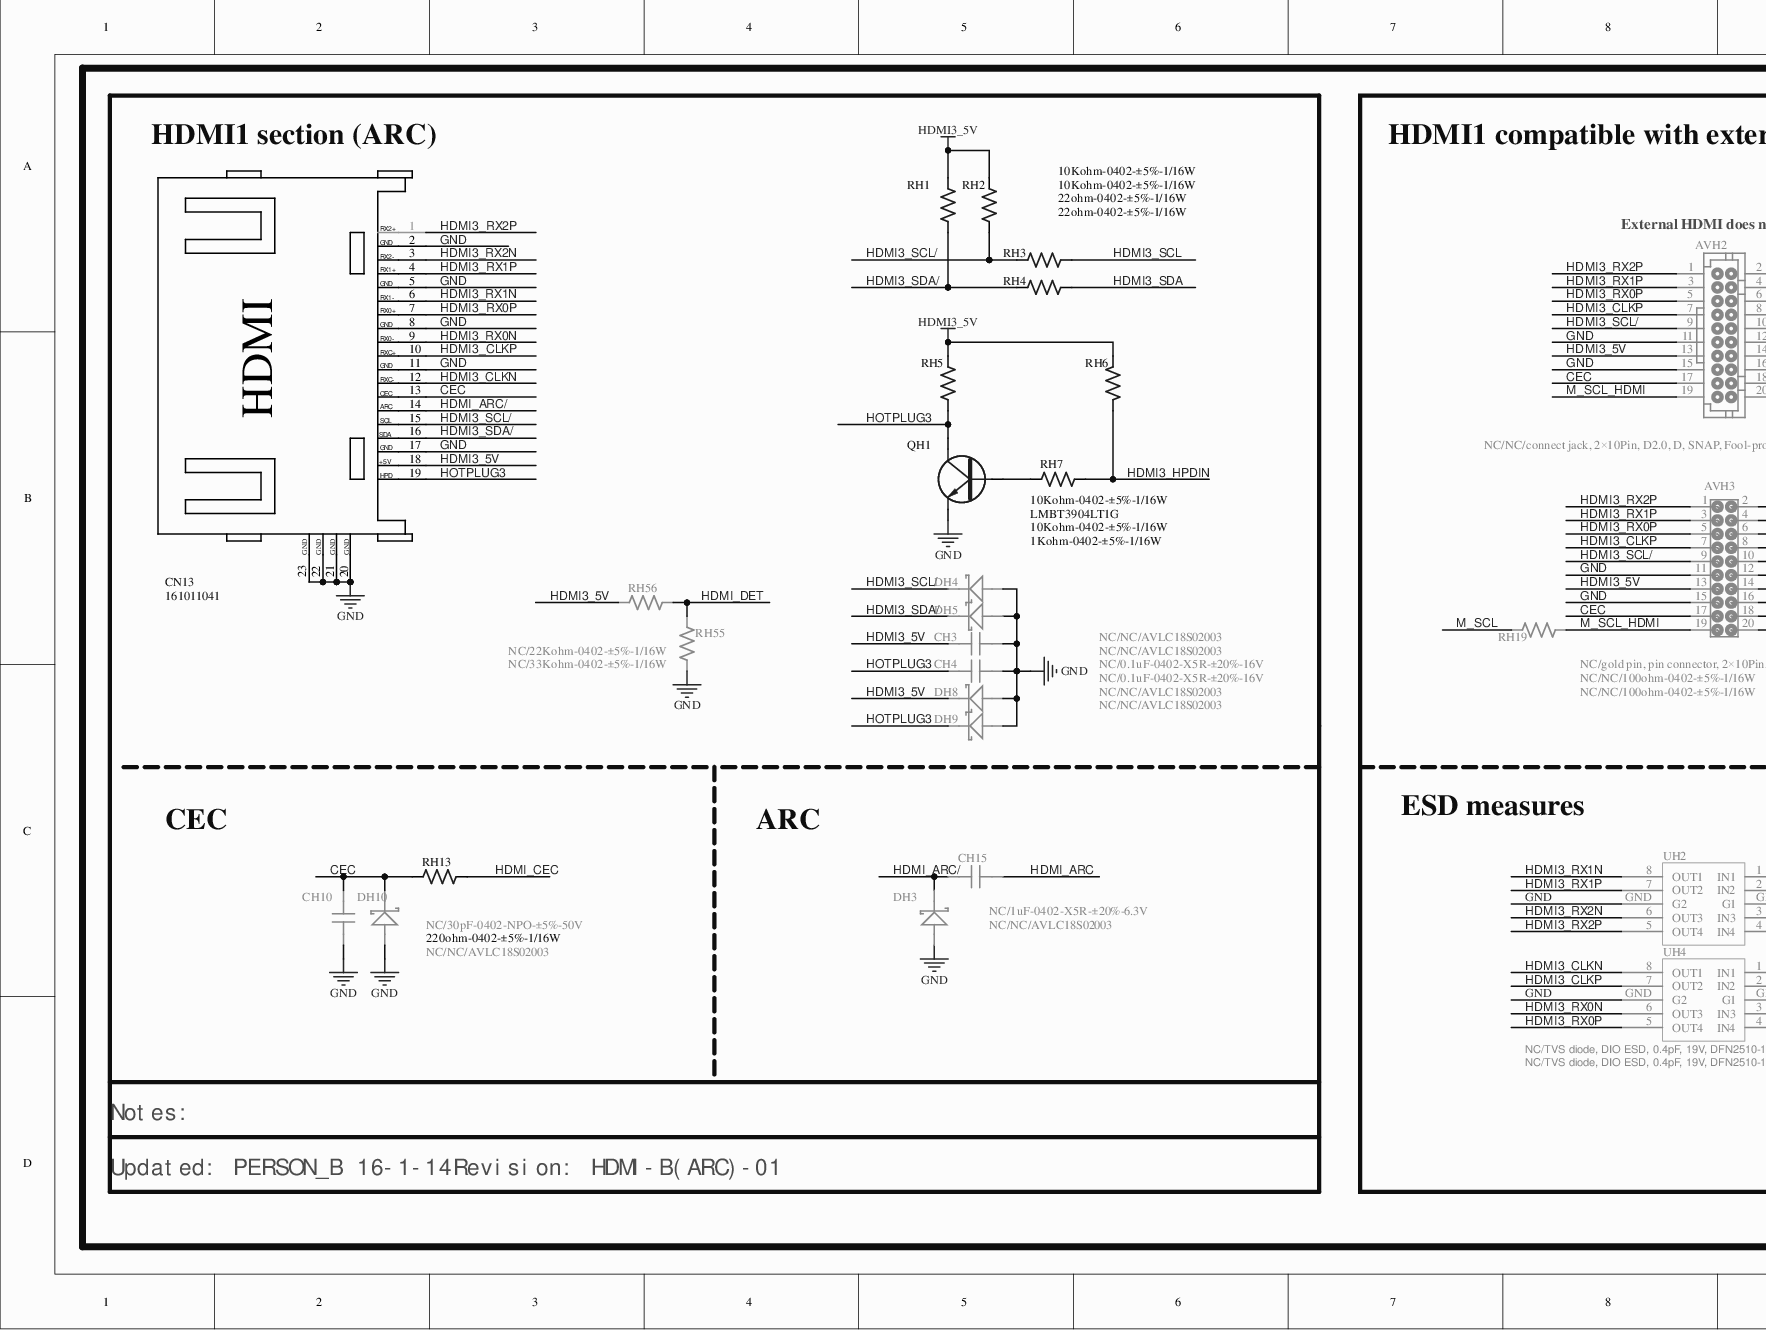
[diagram p0: MISC84277-10.SchDoc, left]
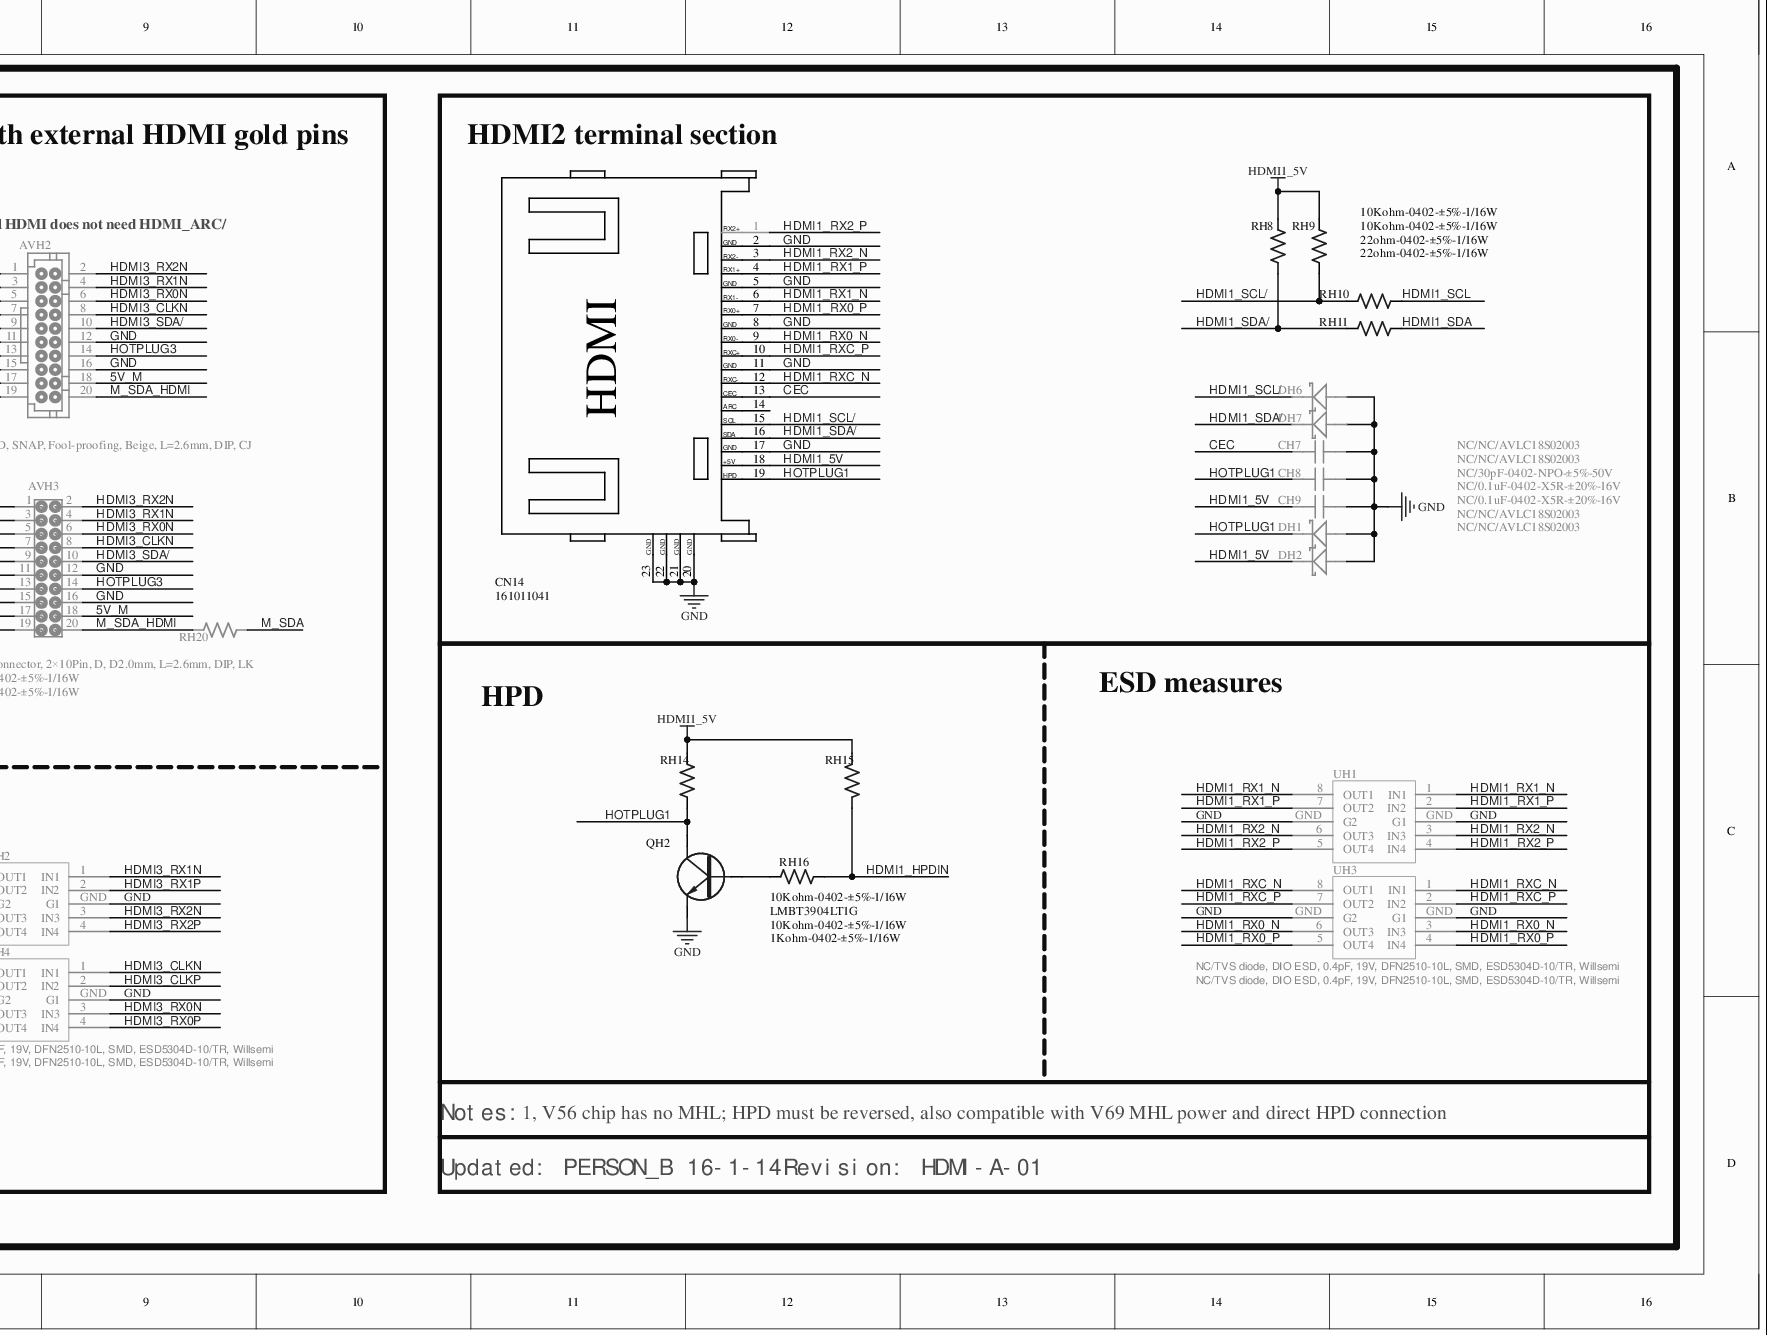
[diagram p1: MISC84277-10.SchDoc, right]
# Altium project MISC84277-14.PrjPCB (part 9 of 10)

## Sheet MISC84277-10.SchDoc
size 635 x 246 mm

### Parts
AVH2  NC/NC/connect jack, 2×10Pin, D2.0, D, SNAP, Fool-proofing, Beige, L=2.6mm, DIP, CJ  [SIP2*10/2.0D-4]
AVH3  NC/gold pin, pin connector, 2×10Pin, D, D2.0mm, L=2.6mm, DIP, LK  [SIP2*10/2.0DM-1]
CH3  NC/0.1uF-0402-X5R-±20%-16V  [C0402]
CH4  NC/0.1uF-0402-X5R-±20%-16V  [C0402]
CH7  NC/30pF-0402-NPO-±5%-50V  [C0402]
CH8  NC/0.1uF-0402-X5R-±20%-16V  [C0402]
CH9  NC/0.1uF-0402-X5R-±20%-16V  [C0402]
CH10  NC/30pF-0402-NPO-±5%-50V  [C0402]
CH15  NC/1uF-0402-X5R-±20%-6.3V  [C0402]
CN13  161011041  [HDMI-HS-1]
CN14  161011041  [HDMI-HS-1]
DH1  NC/NC/AVLC18S02003  [DIODE-S0402]
DH2  NC/NC/AVLC18S02003  [DIODE-S0402]
DH3  NC/NC/AVLC18S02003  [DIODE-S0402]
DH4  NC/NC/AVLC18S02003  [DIODE-S0402]
DH5  NC/NC/AVLC18S02003  [DIODE-S0402]
DH6  NC/NC/AVLC18S02003  [DIODE-S0402]
DH7  NC/NC/AVLC18S02003  [DIODE-S0402]
DH8  NC/NC/AVLC18S02003  [DIODE-S0402]
DH9  NC/NC/AVLC18S02003  [DIODE-S0402]
DH10  NC/NC/AVLC18S02003  [DIODE-S0402]
QH1  LMBT3904LT1G  [SOT-23]
QH2  LMBT3904LT1G  [SOT-23]
RH1  10Kohm-0402-±5%-1/16W  [R0402]
RH2  10Kohm-0402-±5%-1/16W  [R0402]
RH3  22ohm-0402-±5%-1/16W  [R0402]
RH4  22ohm-0402-±5%-1/16W  [R0402]
RH5  1Kohm-0402-±5%-1/16W  [R0402]
RH6  10Kohm-0402-±5%-1/16W  [R0402]
RH7  10Kohm-0402-±5%-1/16W  [R0402]
RH8  10Kohm-0402-±5%-1/16W  [R0402]
RH9  10Kohm-0402-±5%-1/16W  [R0402]
RH10  22ohm-0402-±5%-1/16W  [R0402]
RH11  22ohm-0402-±5%-1/16W  [R0402]
RH13  220ohm-0402-±5%-1/16W  [R0402]
RH14  1Kohm-0402-±5%-1/16W  [R0402]
RH15  10Kohm-0402-±5%-1/16W  [R0402]
RH16  10Kohm-0402-±5%-1/16W  [R0402]
RH19  NC/NC/100ohm-0402-±5%-1/16W  [R0402]
RH20  NC/NC/100ohm-0402-±5%-1/16W  [R0402]
RH55  NC/33Kohm-0402-±5%-1/16W  [R0402]
RH56  NC/22Kohm-0402-±5%-1/16W  [R0402]
UH1  NC/TVS diode, DIO ESD, 0.4pF, 19V, DFN2510-10L, SMD, ESD5304D-10/TR, Willsemi  [RCL0524P]
UH2  NC/TVS diode, DIO ESD, 0.4pF, 19V, DFN2510-10L, SMD, ESD5304D-10/TR, Willsemi  [RCL0524P]
UH3  NC/TVS diode, DIO ESD, 0.4pF, 19V, DFN2510-10L, SMD, ESD5304D-10/TR, Willsemi  [RCL0524P]
UH4  NC/TVS diode, DIO ESD, 0.4pF, 19V, DFN2510-10L, SMD, ESD5304D-10/TR, Willsemi  [RCL0524P]

### Blocks framed on the sheet
HDMI2 terminal section: CH7-CH9 CN14 DH1 DH2 DH6 DH7 RH8-RH11

### Nets
5V_M: AVH2.18 AVH3.18
GND: AVH2.11 AVH2.12 AVH2.15 AVH2.16 AVH3.11 AVH3.12 AVH3.15 AVH3.16 CH3.1 CH4.1 CH7.1 CH8.1 CH9.1 CH10.1 CN13.2 CN13.5 CN13.8 CN13.11 CN13.17 CN13.20 CN13.21 CN13.22 CN13.23 CN14.2 CN14.5 CN14.8 CN14.11 CN14.17 CN14.20 CN14.21 CN14.22 CN14.23 DH1.A DH2.A DH3.A DH4.A DH5.A DH6.A DH7.A DH8.A DH9.A DH10.A QH1.E QH2.E RH55.2 UH1.GND(G1) UH2.GND(G1) UH3.GND(G1) UH4.GND(G1)
HDMI1_5V: CH9.2 CN14.18 DH2.K RH8.2 RH9.2 RH14.2 RH15.1
HDMI3_5V: AVH2.13 AVH3.13 CH3.2 CN13.18 DH8.K RH1.2 RH2.2 RH5.2 RH6.1 RH56.2
CEC: AVH2.17 AVH3.17 CH7.2 CH10.2 CN13.13 CN14.13 DH10.K RH13.2
HDMI1_HPDIN: RH15.2 RH16.2
HDMI1_RX0_N: CN14.9 UH3.3(IN3) UH3.6(OUT3)
HDMI1_RX0_P: CN14.7 UH3.4(IN4) UH3.5(OUT4)
HDMI1_RX1_N: CN14.6 UH1.1(IN1) UH1.8(OUT1)
HDMI1_RX1_P: CN14.4 UH1.2(IN2) UH1.7(OUT2)
HDMI1_RX2_N: CN14.3 UH1.3(IN3) UH1.6(OUT3)
HDMI1_RX2_P: CN14.1 UH1.4(IN4) UH1.5(OUT4)
HDMI1_RXC_N: CN14.12 UH3.1(IN1) UH3.8(OUT1)
HDMI1_RXC_P: CN14.10 UH3.2(IN2) UH3.7(OUT2)
HDMI1_SCL: RH10.1
HDMI1_SCL/: CN14.15 DH6.K RH9.1 RH10.2
HDMI1_SDA: RH11.1
HDMI1_SDA/: CN14.16 DH7.K RH8.1 RH11.2
HDMI3_CLKN: AVH2.8 AVH3.8 CN13.12 UH4.1(IN1) UH4.8(OUT1)
HDMI3_CLKP: AVH2.7 AVH3.7 CN13.10 UH4.2(IN2) UH4.7(OUT2)
HDMI3_HPDIN: RH6.2 RH7.2
HDMI3_RX0N: AVH2.6 AVH3.6 CN13.9 UH4.3(IN3) UH4.6(OUT3)
HDMI3_RX0P: AVH2.5 AVH3.5 CN13.7 UH4.4(IN4) UH4.5(OUT4)
HDMI3_RX1N: AVH2.4 AVH3.4 CN13.6 UH2.1(IN1) UH2.8(OUT1)
HDMI3_RX1P: AVH2.3 AVH3.3 CN13.4 UH2.2(IN2) UH2.7(OUT2)
HDMI3_RX2N: AVH2.2 AVH3.2 CN13.3 UH2.3(IN3) UH2.6(OUT3)
HDMI3_RX2P: AVH2.1 AVH3.1 CN13.1 UH2.4(IN4) UH2.5(OUT4)
HDMI3_SCL: RH3.1
HDMI3_SCL/: AVH2.9 AVH3.9 CN13.15 DH4.K RH2.1 RH3.2
HDMI3_SDA: RH4.1
HDMI3_SDA/: AVH2.10 AVH3.10 CN13.16 DH5.K RH1.1 RH4.2
HDMI_ARC: CH15.1
HDMI_ARC/: CH15.2 CN13.14 DH3.K
HDMI_CEC: RH13.1
HDMI_DET: RH55.1 RH56.1
HOTPLUG1: CH8.2 CN14.19 DH1.K QH2.C RH14.1
HOTPLUG3: AVH2.14 AVH3.14 CH4.2 CN13.19 DH9.K QH1.C RH5.1
M_SCL: RH19.1
M_SCL_HDMI: AVH2.19 AVH3.19 RH19.2
M_SDA: RH20.1
M_SDA_HDMI: AVH2.20 AVH3.20 RH20.2
NetQH1_B: QH1.B RH7.1
NetQH2_B: QH2.B RH16.1

Not connected (* = marked no-connect by the designer): CN14 14*

### Notes on the sheet
- HDMI1 section (ARC)
- HDMI1 compatible with external HDMI gold pins
- (near AVH2) External HDMI does not need HDMI_ARC/
- HPD
- ESD measures
- CEC
- ARC
- Notes:
- 1, V56 chip has no MHL; HPD must be reversed, also compatible with V69 MHL power and direct HPD connection
- Updated: PERSON_B 16-1-14
- Revision: HDMI-B(ARC)-01
- Revision: HDMI-A-01

### Library data of the parts
AVH2 = 连接插座,connect jack,2×10Pin,D2.0,D,SNAP,Fool-proofing,Beige,L=2.6mm,DIP,CJ-DHMI: CN-latched
AVH3 = 2*10PIN-2.0-D-H-M-DHMI: CN-straight gold pin
CH3 CH7 CH10 = 33pF-0402-NPO-±5%-50V-D
CH4 CH8 CH9 CH15 = 0.1uF-0402-Y5V-+80%-20%-16V-D
CN13 CN14 = 161031041(外壳SPCC)-D: CN-HDMI-horizontal-#-#
DH1-DH10 = AVLC18S02003-D
QH1 QH2 = MMBT3904(f≥350MHz)-D-NPN: Q-NPN-#-#-#
RH1-RH4 RH6-RH11 RH15 RH16 = 10Kohm-0402-±5%-1/16W-D
RH5 RH14 = 1Kohm-0402-±5%-1/16W-D
RH13 = 220ohm-0402-±5%-1/16W-D
RH19 RH20 = 100ohm-0402-±5%-1/16W-D
RH55 = 33Kohm-0402-±5%-1/16W-D
RH56 = 22Kohm-0402-±5%-1/16W-D
UH1-UH4 = ULC0524P-D: RCLAMP0524J

## Sheet MISC84277-11.SchDoc
size 393 x 243 mm
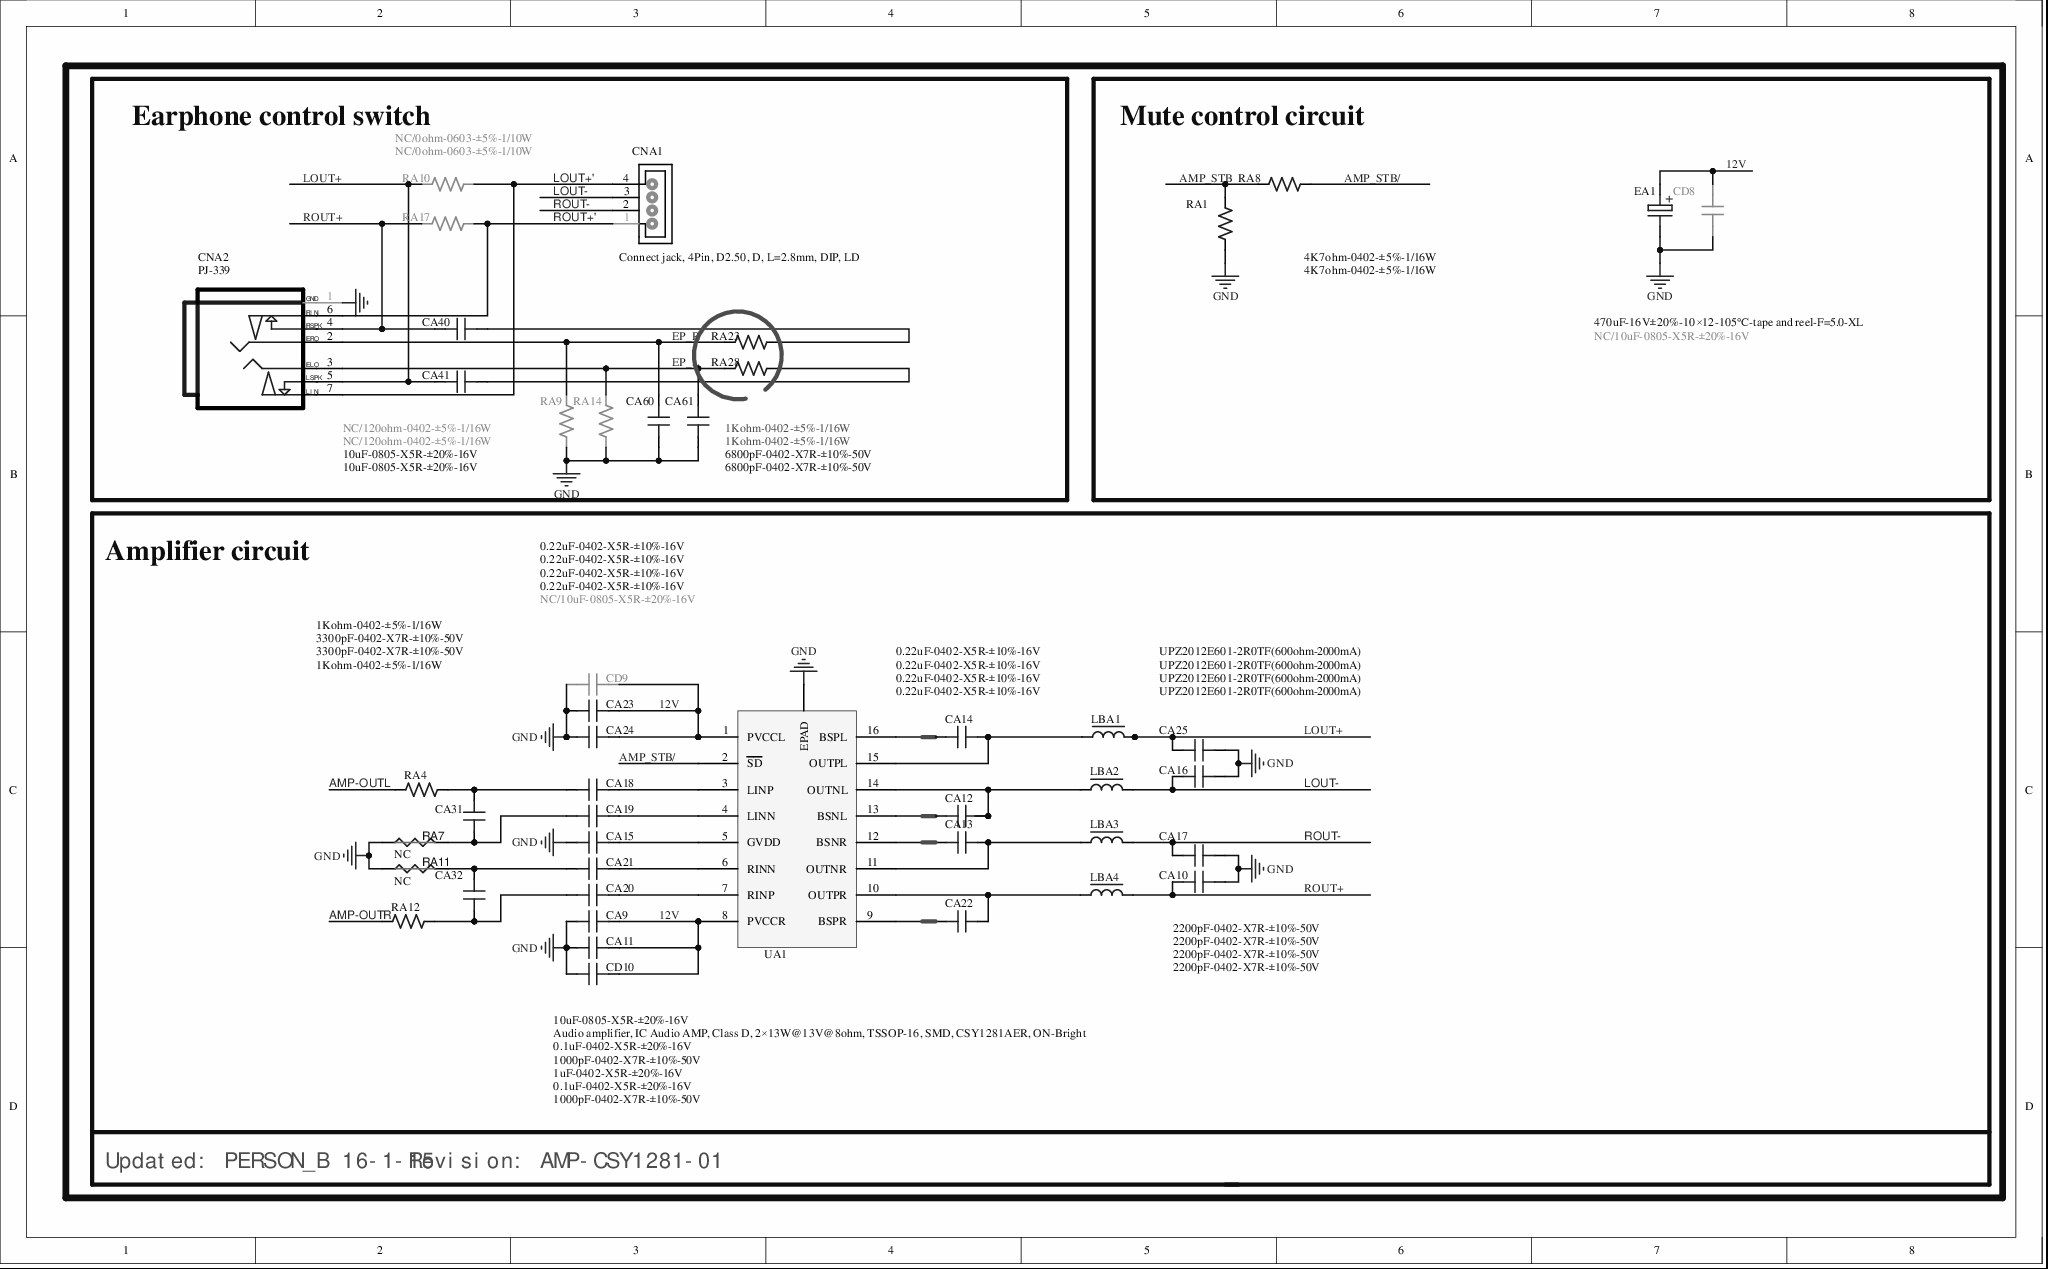
[diagram p2: MISC84277-11.SchDoc]

### Parts
CA9  1000pF-0402-X7R-±10%-50V  [C0402]
CA10  2200pF-0402-X7R-±10%-50V  [C0402]
CA11  0.1uF-0402-X5R-±20%-16V  [C0402]
CA12  0.22uF-0402-X5R-±10%-16V  [C0402]
CA13  0.22uF-0402-X5R-±10%-16V  [C0402]
CA14  0.22uF-0402-X5R-±10%-16V  [C0402]
CA15  1uF-0402-X5R-±20%-16V  [C0402]
CA16  2200pF-0402-X7R-±10%-50V  [C0402]
CA17  2200pF-0402-X7R-±10%-50V  [C0402]
CA18  0.22uF-0402-X5R-±10%-16V  [C0402]
CA19  0.22uF-0402-X5R-±10%-16V  [C0402]
CA20  0.22uF-0402-X5R-±10%-16V  [C0402]
CA21  0.22uF-0402-X5R-±10%-16V  [C0402]
CA22  0.22uF-0402-X5R-±10%-16V  [C0402]
CA23  0.1uF-0402-X5R-±20%-16V  [C0402]
CA24  1000pF-0402-X7R-±10%-50V  [C0402]
CA25  2200pF-0402-X7R-±10%-50V  [C0402]
CA31  3300pF-0402-X7R-±10%-50V  [C0402]
CA32  3300pF-0402-X7R-±10%-50V  [C0402]
CA40  10uF-0805-X5R-±20%-16V  [C0805]
CA41  10uF-0805-X5R-±20%-16V  [C0805]
CA60  6800pF-0402-X7R-±10%-50V  [C0402]
CA61  6800pF-0402-X7R-±10%-50V  [C0402]
CD8  NC/10uF-0805-X5R-±20%-16V  [C0805]
CD9  NC/10uF-0805-X5R-±20%-16V  [C0805]
CD10  10uF-0805-X5R-±20%-16V  [C0805]
CNA1  Connect jack, 4Pin, D2.50, D, L=2.8mm, DIP, LD  [SIP4/2.54D-1]
CNA2  PJ-339  [PHONE-HD-12]
EA1  470uF-16V±20%-10×12-105℃-tape and reel-F=5.0-XL  [EC(10*12)-V-5]
LBA1  UPZ2012E601-2R0TF(600ohm-2000mA)  [L0805]
LBA2  UPZ2012E601-2R0TF(600ohm-2000mA)  [L0805]
LBA3  UPZ2012E601-2R0TF(600ohm-2000mA)  [L0805]
LBA4  UPZ2012E601-2R0TF(600ohm-2000mA)  [L0805]
RA1  4K7ohm-0402-±5%-1/16W  [R0402]
RA4  1Kohm-0402-±5%-1/16W  [R0402]
RA7  NC  [GND]
RA8  4K7ohm-0402-±5%-1/16W  [R0402]
RA9  NC/120ohm-0402-±5%-1/16W  [R0402]
RA10  NC/0ohm-0603-±5%-1/10W  [R0603]
RA11  NC  [GND]
RA12  1Kohm-0402-±5%-1/16W  [R0402]
RA14  NC/120ohm-0402-±5%-1/16W  [R0402]
RA17  NC/0ohm-0603-±5%-1/10W  [R0603]
RA23  1Kohm-0402-±5%-1/16W  [R0402]
RA28  1Kohm-0402-±5%-1/16W  [R0402]
UA1  Audio amplifier, IC Audio AMP, Class D, 2×13W@13V@8ohm, TSSOP-16, SMD, CSY1281AER, ON-Bright  [SOP16/1.27-7]

### Blocks framed on the sheet
Earphone control switch: CA40 CA41 CA60 CA61 CNA1 CNA2 RA9 RA10 RA14 RA17 RA23 RA28
Mute control circuit: CD8 EA1 RA1 RA8

### Nets
12V: CA9.1 CA11.1 CA23.1 CA24.1 CD8.1 CD9.2 CD10.2 EA1.1 UA1.1(PVCCL) UA1.8(PVCCR)
GND: CA9.2 CA10.2 CA11.2 CA15.1 CA16.1 CA17.2 CA23.2 CA24.2 CA25.2 CA60.2 CA61.2 CD8.2 CD9.1 CD10.1 CNA2.1 EA1.2 RA1.1 RA7.JP_2K RA9.1 RA11.JP_2K RA14.1 UA1.EPAD
AMP-OUTL: RA4.1
AMP-OUTR: RA12.1
AMP_STB: RA1.2 RA8.1
AMP_STB/: RA8.2 UA1.2(~{SD})
EP_L: CA61.1 CNA2.3 RA14.2 RA28.1
EP_R: CA60.1 CNA2.2 RA9.2 RA23.1
LOUT+: CA25.1 CA41.2 CNA2.5 LBA1.2 RA10.1
LOUT+': CNA1.4 CNA2.7 RA10.2
LOUT-: CA16.2 CNA1.3 LBA2.2
ROUT+: CA10.1 CA40.2 CNA2.4 LBA4.2 RA17.1
ROUT+': CNA1.1 CNA2.6 RA17.2
ROUT-: CA17.1 CNA1.2 LBA3.2
NetCA12_1: CA12.1 UA1.13(BSNL)
NetCA12_2: CA12.2 LBA2.1 UA1.14(OUTNL)
NetCA13_1: CA13.1 UA1.12(BSNR)
NetCA13_2: CA13.2 LBA3.1 UA1.11(OUTNR)
NetCA14_1: CA14.1 UA1.16(BSPL)
NetCA14_2: CA14.2 LBA1.1 UA1.15(OUTPL)
NetCA15_2: CA15.2 UA1.5(GVDD)
NetCA18_1: CA18.1 UA1.3(LINP)
NetCA18_2: CA18.2 CA31.2 RA4.2
NetCA19_1: CA19.1 UA1.4(LINN)
NetCA19_2: CA19.2 CA31.1 RA7.JP_1K
NetCA20_1: CA20.1 UA1.7(RINP)
NetCA20_2: CA20.2 CA32.1 RA12.2
NetCA21_1: CA21.1 UA1.6(RINN)
NetCA21_2: CA21.2 CA32.2 RA11.JP_1K
NetCA22_1: CA22.1 UA1.9(BSPR)
NetCA22_2: CA22.2 LBA4.1 UA1.10(OUTPR)
NetCA40_1: CA40.1 RA23.2
NetCA41_1: CA41.1 RA28.2

### Notes on the sheet
- Amplifier circuit
- Updated: PERSON_B 16-1-15
- Revision: AMP-CSY1281-01

### Library data of the parts
CA9 CA10 CA16 CA17 CA24 CA25 = 1000pF-0402-X7R-±10%-50V-D
CA11 CA23 = 0.1uF-0402-X5R-±20%-16V-D
CA12-CA14 CA18-CA22 = 0.22uF-0402-X5R-±10%-16V-D
CA15 = 1uF-0402-X5R-±20%-16V-D
CA31 CA32 = 3300pF-0402-X7R-±10%-50V-D
CA40 CA41 CD8-CD10 = 10uF-0805-X5R-±20%-16V-D
CA60 CA61 = 0.022uF-0402-X7R-±10%-16V-D
CNA1 = 4PIN-2.54-D-H-G-DHMI
CNA2 = PJ-339-DLMI-headphone: CN-headphone-#-#-#
EA1 = 470uF-16V±20%-10×12-105℃-编带-F=5.0-XL-DHAI
LBA1-LBA4 = 300ohm-2500mA-0805-D
RA1 RA8 = 100ohm-0402-±5%-1/16W-D
RA4 RA12 = 1Kohm-0402-±5%-1/16W-D
RA7 RA11 = GND: Manufacturer: Panasonic; Part Number: ERJ3GEYJ473V; Right: 20; Bottom: 30; CLASS: Discrete; Comments: Digikey
RA9 RA14 = 330ohm-0402-±5%-1/16W-D
RA10 RA17 = 0ohm-0603-±5%-1/10W-D
RA23 RA28 = 1kohm-0402-±5%-1/16W-D
UA1 = 音频功放,IC Audio AMP,Class D,2×13W@13.0V@8ohm,TSSOP16,SMD,OB6223BPA,On-bright-D